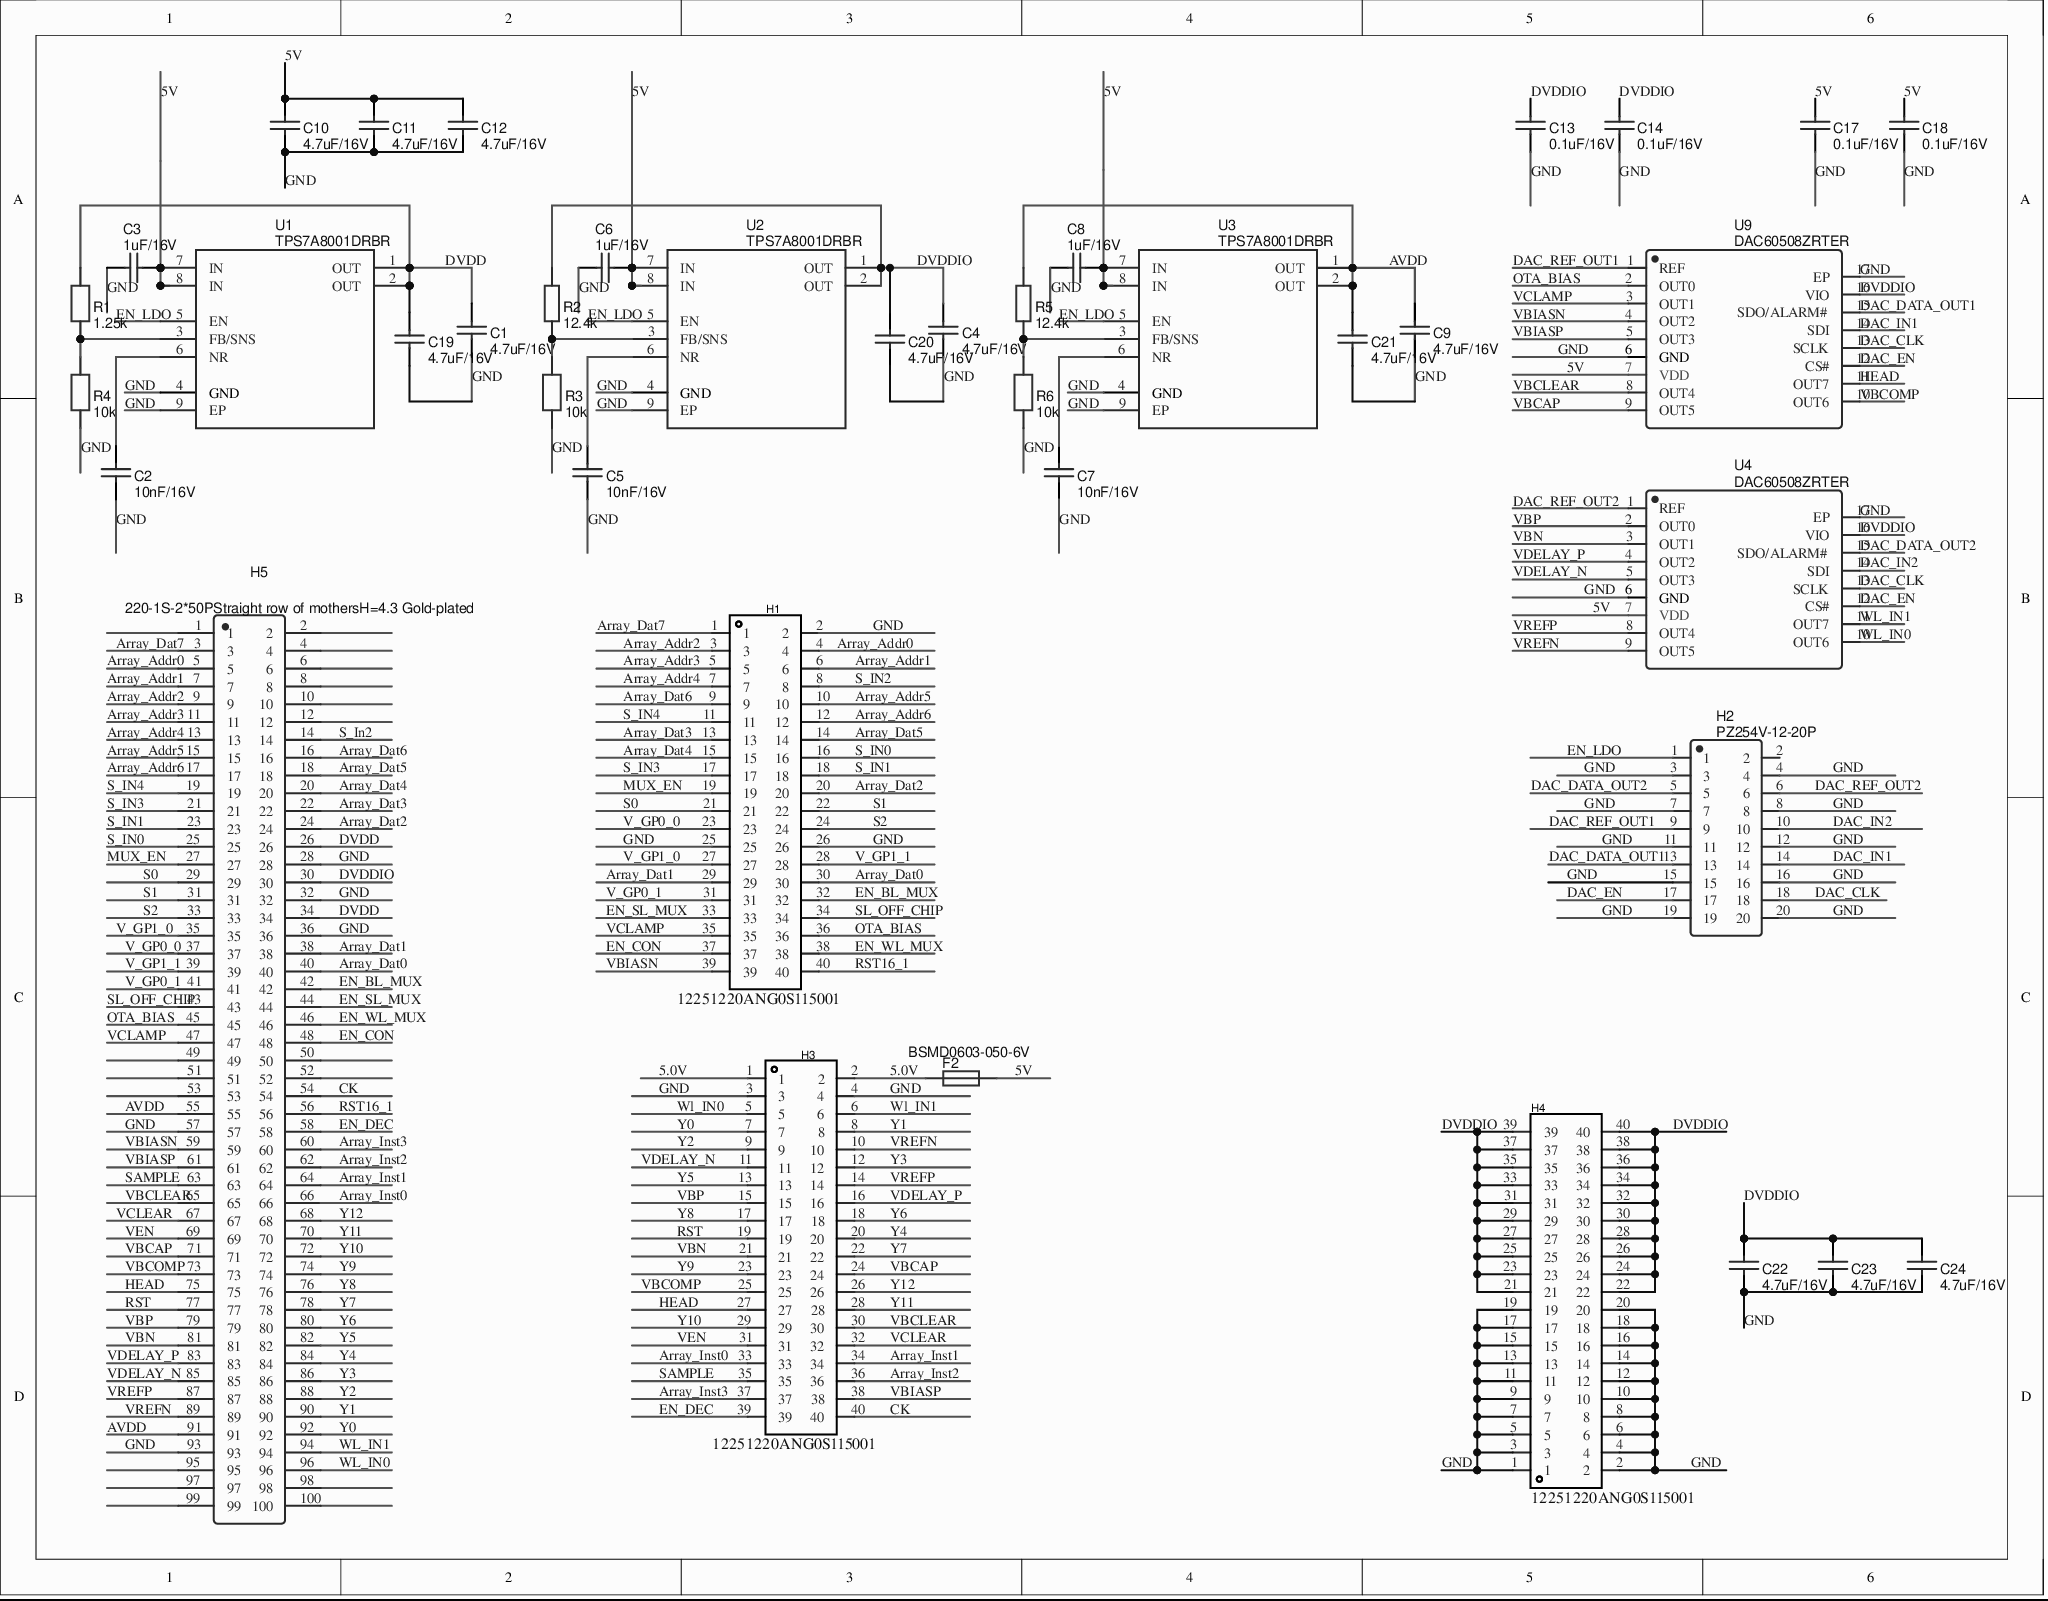
[diagram p0: MISC62795-4.schdoc]
# Altium project MISC62795-7.PrjPCB
1 sheet, 39 parts. Net scope: global (net labels, ports and power ports of the same name join across sheets).
Board file: MISC62795.pcbdoc

## Sheet MISC62795-4.schdoc
size 291 x 227 mm

### Parts
C1  4.7uF/16V  [C0603]
C2  10nF/16V  [C0603]
C3  1uF/16V  [C0603]
C4  4.7uF/16V  [C0603]
C5  10nF/16V  [C0603]
C6  1uF/16V  [C0603]
C7  10nF/16V  [C0603]
C8  1uF/16V  [C0603]
C9  4.7uF/16V  [C0603]
C10  4.7uF/16V  [C0603]
C11  4.7uF/16V  [C0603]
C12  4.7uF/16V  [C0603]
C13  0.1uF/16V  [C0603]
C14  0.1uF/16V  [C0603]
C17  0.1uF/16V  [C0603]
C18  0.1uF/16V  [C0603]
C19  4.7uF/16V  [C0603]
C20  4.7uF/16V  [C0603]
C21  4.7uF/16V  [C0603]
C22  4.7uF/16V  [C0603]
C23  4.7uF/16V  [C0603]
C24  4.7uF/16V  [C0603]
F2  BSMD0603-050-6V  [F0603]
H1  12251220ANG0S115001  [HDR-TH_40P-P2.54-V-M-R2-C20-S2.54]
H2  PZ254V-12-20P  [HDR-TH_20P-P2.54-V-M-R2-C10-S2.54]
H3  12251220ANG0S115001  [HDR-TH_40P-P2.54-V-M-R2-C20-S2.54]
H4  12251220ANG0S115001  [HDR-TH_40P-P2.54-V-M-R2-C20-S2.54]
H5  220-1S-2*50PStraight row of mothersH=4.3 Gold-plated  [IC51-1004-809-23]
R1  1.25k  [R0805]
R2  12.4k  [R0805]
R3  10k  [R0805]
R4  10k  [R0805]
R5  12.4k  [R0805]
R6  10k  [R0805]
U1  TPS7A8001DRBR  [VSON-8_L3.0-W3.0-P0.65-TL-EP]
U2  TPS7A8001DRBR  [VSON-8_L3.0-W3.0-P0.65-TL-EP]
U3  TPS7A8001DRBR  [VSON-8_L3.0-W3.0-P0.65-TL-EP]
U4  DAC60508ZRTER  [WQFN-16_L3.0-W3.0-P0.50-BL-EP0.8]
U9  DAC60508ZRTER  [WQFN-16_L3.0-W3.0-P0.50-BL-EP0.8]

### Nets
5.0V: F2.2 H3.1 H3.2
5V: C3.1 C6.1 C8.1 C10.2 C11.2 C12.2 C17.2 C18.2 F2.1 U1.7(IN) U1.8(IN) U2.7(IN) U2.8(IN) U3.7(IN) U3.8(IN) U4.7(VDD) U9.7(VDD)
Array_Addr0: H1.4 H5.5
Array_Addr1: H1.6 H5.7
Array_Addr2: H1.3 H5.9
Array_Addr3: H1.5 H5.11
Array_Addr4: H1.7 H5.13
Array_Addr5: H1.10 H5.15
Array_Addr6: H1.12 H5.17
Array_Dat0: H1.30 H5.40
Array_Dat1: H1.29 H5.38
Array_Dat2: H1.20 H5.24
Array_Dat3: H1.13 H5.22
Array_Dat4: H1.15 H5.20
Array_Dat5: H1.14 H5.18
Array_Dat6: H1.9 H5.16
Array_Dat7: H1.1 H5.3
Array_Inst0: H3.33 H5.66
Array_Inst1: H3.34 H5.64
Array_Inst2: H3.36 H5.62
Array_Inst3: H3.37 H5.60
AVDD: C9.2 C21.2 H5.55 H5.91 R5.1 U3.1(OUT) U3.2(OUT)
CK: H3.40 H5.54
DAC_CLK: H2.18 U4.13(SCLK) U9.13(SCLK)
DAC_DATA_OUT1: H2.13 U9.15(SDO/ALARM#)
DAC_DATA_OUT2: H2.5 U4.15(SDO/ALARM#)
DAC_EN: H2.17 U4.12(CS#) U9.12(CS#)
DAC_IN1: H2.14 U9.14(SDI)
DAC_IN2: H2.10 U4.14(SDI)
DAC_REF_OUT1: H2.9 U9.1(REF)
DAC_REF_OUT2: H2.6 U4.1(REF)
DVDD: C1.2 C19.2 H5.26 H5.34 R1.1 U1.1(OUT) U1.2(OUT)
DVDDIO: C4.2 C13.2 C14.2 C20.2 C22.2 C23.2 C24.2 H4.21 H4.22 H4.23 H4.24 H4.25 H4.26 H4.27 H4.28 H4.29 H4.30 H4.31 H4.32 H4.33 H4.34 H4.35 H4.36 H4.37 H4.38 H4.39 H4.40 H5.30 R2.1 U2.1(OUT) U2.2(OUT) U4.16(VIO) U9.16(VIO)
EN_BL_MUX: H1.32 H5.42
EN_CON: H1.37 H5.48
EN_DEC: H3.39 H5.58
EN_LDO: H2.1 U1.5(EN) U2.5(EN) U3.5(EN)
EN_SL_MUX: H1.33 H5.44
EN_WL_MUX: H1.38 H5.46
GND: C1.1 C2.1 C3.2 C4.1 C5.1 C6.2 C7.1 C8.2 C9.1 C10.1 C11.1 C12.1 C13.1 C14.1 C17.1 C18.1 C19.1 C20.1 C21.1 C22.1 C23.1 C24.1 H1.2 H1.25 H1.26 H2.3 H2.4 H2.7 H2.8 H2.11 H2.12 H2.15 H2.16 H2.19 H2.20 H3.3 H3.4 H4.1 H4.2 H4.3 H4.4 H4.5 H4.6 H4.7 H4.8 H4.9 H4.10 H4.11 H4.12 H4.13 H4.14 H4.15 H4.16 H4.17 H4.18 H4.19 H4.20 H5.28 H5.32 H5.36 H5.57 H5.93 R3.1 R4.1 R6.1 U1.4(GND) U1.9(EP) U2.4(GND) U2.9(EP) U3.4(GND) U3.9(EP) U4.6(GND) U4.17(EP) U9.6(GND) U9.17(EP)
HEAD: H3.27 H5.75 U9.11(OUT7)
MUX_EN: H1.19 H5.27
OTA_BIAS: H1.36 H5.45 U9.2(OUT0)
RST: H3.19 H5.77
RST16_1: H1.40 H5.56
S0: H1.21 H5.29
S1: H1.22 H5.31
S2: H1.24 H5.33
S_IN0: H1.16 H5.25
S_IN1: H1.18 H5.23
S_In2: H1.8 H5.14
S_IN3: H1.17 H5.21
S_IN4: H1.11 H5.19
SAMPLE: H3.35 H5.63
SL_OFF_CHIP: H1.34 H5.43
V_GP0_0: H1.23 H5.37
V_GP0_1: H1.31 H5.41
V_GP1_0: H1.27 H5.35
V_GP1_1: H1.28 H5.39
VBCAP: H3.24 H5.71 U9.9(OUT5)
VBCLEAR: H3.30 H5.65 U9.8(OUT4)
VBCOMP: H3.25 H5.73 U9.10(OUT6)
VBIASN: H1.39 H5.59 U9.4(OUT2)
VBIASP: H3.38 H5.61 U9.5(OUT3)
VBN: H3.21 H5.81 U4.3(OUT1)
VBP: H3.15 H5.79 U4.2(OUT0)
VCLAMP: H1.35 H5.47 U9.3(OUT1)
VCLEAR: H3.32 H5.67
VDELAY_N: H3.11 H5.85 U4.5(OUT3)
VDELAY_P: H3.16 H5.83 U4.4(OUT2)
VEN: H3.31 H5.69
VREFN: H3.10 H5.89 U4.9(OUT5)
VREFP: H3.14 H5.87 U4.8(OUT4)
WL_IN0: H3.5 H5.96 U4.10(OUT6)
WL_IN1: H3.6 H5.94 U4.11(OUT7)
Y0: H3.7 H5.92
Y1: H3.8 H5.90
Y2: H3.9 H5.88
Y3: H3.12 H5.86
Y4: H3.20 H5.84
Y5: H3.13 H5.82
Y6: H3.18 H5.80
Y7: H3.22 H5.78
Y8: H3.17 H5.76
Y9: H3.23 H5.74
Y10: H3.29 H5.72
Y11: H3.28 H5.70
Y12: H3.26 H5.68
NetC2_2: C2.2 U1.6(NR)
NetC5_2: C5.2 U2.6(NR)
NetC7_2: C7.2 U3.6(NR)
NetR1_2: R1.2 R4.2 U1.3(FB/SNS)
NetR2_2: R2.2 R3.2 U2.3(FB/SNS)
NetR5_2: R5.2 R6.2 U3.3(FB/SNS)

Not connected (* = marked no-connect by the designer): H2 2; H5 1 2 4 6 8 10 12 49 50 51 52 53 95 97 98 99 100

### Library data of the parts
C1 C4 C9-C12 C19-C24 = 4.7uF: Manufacturer Part: CL10A475KO8NNNC; nameAlias: Value; Supplier: LCSC; Supplier Part: C19666; JLCPCB Part Class: Basic Part; spicePre: C; spiceSymbolName: CL10A475KO8NNNC
C2 C5 C7 C13 C14 C17 C18 = 10nF: Manufacturer Part: CC0603KRX7R9BB103; nameAlias: Value; Supplier: LCSC; Supplier Part: C100042; JLCPCB Part Class: Extended Part; spicePre: C; spiceSymbolName: CC0603KRX7R9BB103
C3 C6 C8 = 1uF: Manufacturer Part: CL10A105KB8NNNC; nameAlias: Value; Supplier: LCSC; Supplier Part: C15849; JLCPCB Part Class: Basic Part; spicePre: C; spiceSymbolName: CL10A105KB8NNNC
F2 = BSMD0603-050-6V: Contributor: LCSC; Supplier: LCSC; Supplier Part: C883095; Manufacturer Part: BSMD0603-050-6V; JLCPCB Part Class: Extended Part; spicePre: F; spiceSymbolName: BSMD0603-050-6V
H1 H3 H4 = 12251220ANG0S115001: Add into BOM: yes; Pin Structure: 2x20P; Pitch: 2.54mm; Current Rating (Max): 3A; Symbol: 12251220ANG0S115001; Device: 12251220ANG0S115001; Supplier: LCSC; Supplier Part: C429965; Manufacturer Part: 12251220ANG0S115001; JLCPCB Part Class: Extended Part; Datasheet: https://atta.szlcsc.com/upload/public/pdf/source/20190920/C429965_BC46B4ED575BB92CEF1C6420E537C4AD.pdf; Convert to PCB: yes; Row Spacing: 2.54mm; Number of Pins: 40P; Voltage Rating (Max): -; Length of Mating Pin: 6mm; Insulation Height: 2.5mm; Length of End Connection Pin: 3mm; Contact Plating: -
H2 = PZ254V-12-20P: Contributor: LCSC; Supplier: LCSC; Supplier Part: C492427; Manufacturer Part: PZ254V-12-20P; JLCPCB Part Class: Extended Part; spicePre: H; spiceSymbolName: PZ254V-12-20P
H5 = 220-1S-2*50PStraight row of mothersH=4.3 Gold-plated: Manufacturer Part: B-2201SA0P-B120; Contributor: LCSC; Supplier: LCSC; Supplier Part: C124395; JLCPCB Part Class: Extended Part; spicePre: H; spiceSymbolName: 220-1S-2*50PStraight row of mothersH=4.3 Gold-plated
R1 = (no symbol name): Manufacturer Part: ARG05BTC1251N; nameAlias: Value; Contributor: LCSC; Supplier: LCSC; Supplier Part: C2441197; JLCPCB Part Class: Extended Part; spicePre: R; spiceSymbolName: ARG05BTC1251N
R2 R5 = (no symbol name): nameAlias: Value; Contributor: LCSC; Supplier: LCSC; Supplier Part: C337058; JLCPCB Part Class: Extended Part; spicePre: R
R3 R4 R6 = (no symbol name): Manufacturer Part: ARG05BTC1002; nameAlias: Value; Contributor: LCSC; Supplier: LCSC; Supplier Part: C406725; JLCPCB Part Class: Extended Part; spicePre: R; spiceSymbolName: ARG05BTC1002
U4 U9 = DAC60508ZRTER: Contributor: LCSC; Supplier: LCSC; Supplier Part: C2679476; Manufacturer Part: DAC60508ZRTER; JLCPCB Part Class: Extended Part; spicePre: U; spiceSymbolName: DAC60508ZRTER
U1-U3 = TPS7A8001DRBR: Supplier: LCSC; Manufacturer Part: TPS7A8001DRBR; Supplier Part: C105265; JLCPCB Part Class: Extended Part; spicePre: U; spiceSymbolName: TPS7A8001DRBR